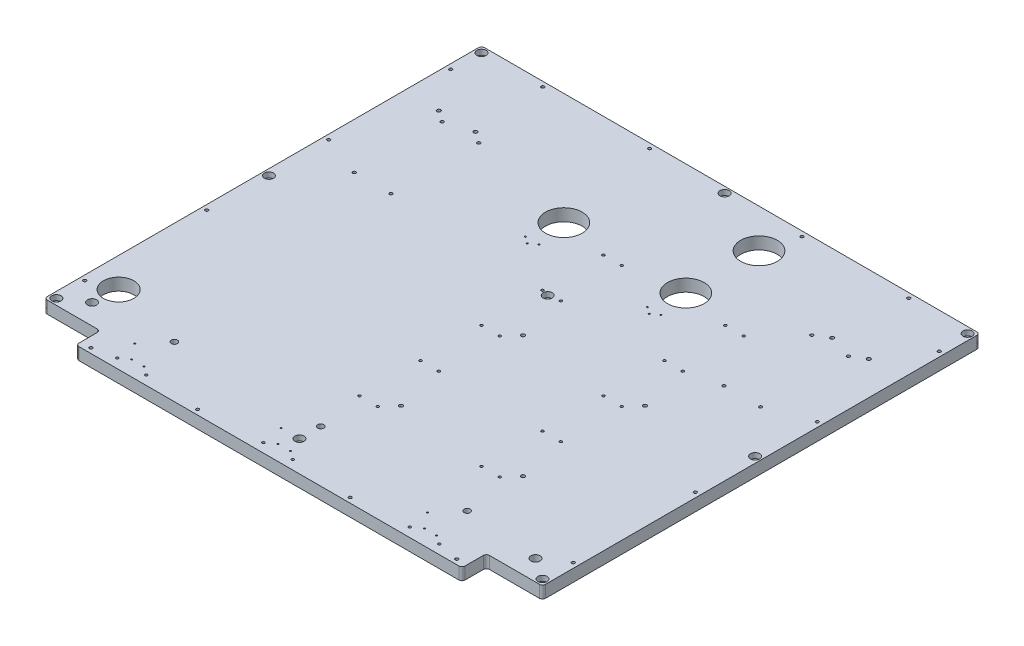
SolidWorks part; units mm, degrees
ref_plane "前视" through (0, 0, 0) normal (0, 0, 1) x (1, 0, 0)
ref_plane "上视" through (0, 0, 0) normal (0, 1, 0) x (1, 0, 0)
ref_plane "右视" through (0, 0, 0) normal (1, 0, 0) x (0, 0, -1)
sketch "草图1" plane through (0, 0, 0) normal (0, 1, 0) x (1, 0, 0)
  line L1 (-425, -375) -> (425, -375)
  line L2 (-425, -375) -> (-425, 375)
  line L3 (-425, 375) -> (425, 375)
  line L4 (425, -375) -> (425, 375)
  line L5 (-425, -375) -> (425, 375) construction
  line L6 (-425, 375) -> (425, -375) construction
  point P0 (0, 0)
  dimension "D1" = 750
  dimension "D2" = 850
extrude "凸台-拉伸1" add sketch "草图1" along normal blind 20
sketch "草图48" plane through (0, 20, 0) normal (0, 1, 0) x (1, 0, 0)
  line L0 (425, 375) -> (-425, 375) construction
  line L2 (425, -375) -> (425, 375) construction
  circle A0 centre (-90, 175) radius 30
  circle A1 centre (110, 175) radius 30
  circle A2 centre (110, 295) radius 30
  dimension "D1" = 200
  dimension "D2" = 315
  dimension "D3" = 60
  dimension "D4" = 200
  dimension "D5" = 80
extrude "切除-拉伸13" cut sketch "草图48" against normal up to next
sketch "草图47" plane through (0, 20, 0) normal (0, 1, 0) x (1, 0, 0)
  line L0 (-425, -375) -> (425, -375) construction
  line L1 (-425, 375) -> (-425, -375) construction
  circle A0 centre (-360, -285) radius 25
  dimension "D1" = 50
  dimension "D2" = 90
  dimension "D3" = 65
extrude "切除-拉伸12" cut sketch "草图47" against normal up to next
sketch "草图37" plane through (0, 20, 0) normal (0, -1, 0) x (-1, 0, 0)
  line L0 (-425, -375) -> (-425, 375) construction
  line L1 (-425, 375) -> (425, 375) construction
  line L2 (425, 375) -> (425, -375) construction
  line L3 (425, -375) -> (-425, -375) construction
  line L4 (-425, -375) -> (-425, 375)
  line L5 (-425, 375) -> (425, 375)
  line L6 (425, 375) -> (425, -375)
  line L7 (425, -375) -> (-425, -375)
  line L8 (-408.5, -358.5) -> (-408.5, 358.5)
  line L9 (-408.5, 358.5) -> (408.5, 358.5)
  line L10 (408.5, 358.5) -> (408.5, -358.5)
  line L11 (408.5, -358.5) -> (-408.5, -358.5)
  dimension "D1" = 16.5
extrude "切除-拉伸10" cut sketch "草图37" along normal through all
sketch "草图38" plane through (0, 20, 0) normal (0, 1, 0) x (1, 0, 0)
  line L1 (-316.5, -398.5) -> (316.5, -398.5)
  line L2 (-316.5, -398.5) -> (-316.5, -358.5)
  line L3 (-316.5, -358.5) -> (316.5, -358.5)
  line L4 (316.5, -398.5) -> (316.5, -358.5)
  line L5 (0, 0) -> (0, 281.3939) construction
  line L6 (408.5, -358.5) -> (-408.5, -358.5) construction
  dimension "D1" = 633
  dimension "D2" = 40
extrude "凸台-拉伸2" add sketch "草图38" against normal up to surface (20 mm away) up to face at (0, 0, 0)
sketch "草图56" plane through (0, 20, 0) normal (0, 1, 0) x (1, 0, 0)
  line L0 (0, 0) -> (0, -181.294) construction
  line L1 (-408.5, -358.5) -> (-408.5, 358.5) construction
  line L3 (-316.5, -358.5) -> (-408.5, -358.5) construction
  circle A0 centre (-363.5, -325) radius 7.5
  circle A1 centre (363.5, -325) radius 7.5
  dimension "D2" = 33.5
  dimension "D3" = 15
  dimension "D1" = 45
extrude "切除-拉伸14" cut sketch "草图56" against normal up to next
hole_wizard "M8 六角凹头螺钉的柱形沉头孔2" positions "草图46" profile "草图45" counterbore size "M8" standard "Iso" end condition through all
sketch "草图46" plane through (0, 20, 0) normal (0, 1, 0) x (1, 0, 0)
  line L0 (0, 0) -> (0, 358.5) construction
  line L4 (0, 0) -> (408.5, 0) construction
  line L6 (408.5, 358.5) -> (408.5, -358.5) construction
  line L7 (-408.5, 358.5) -> (408.5, 358.5) construction
  point P0 (-398.5, 348.5)
  point P2 (-398.5, 0)
  point P4 (-398.5, -348.5)
  point P6 (0, -348.5)
  point P8 (398.5, -348.5)
  point P10 (398.5, 0)
  point P12 (398.5, 348.5)
  point P29 (0, 348.5)
  point P32 (0, 58.5)
  dimension "D1" = 797
  dimension "D2" = 697
  dimension "D3" = 58.5
sketch "草图45" plane through (-398.5, 20, -348.5) normal (1, 0, 0) x (0, 0, 1)
  line L0 (0, 0) -> (0, 20.0001)
  line L1 (0, 20.0001) -> (4.5, 20.0001)
  line L3 (4.5, 20.0001) -> (4.5, 8.6)
  line L4 (4.5, 8.6) -> (7.5, 8.6)
  line L5 (7.5, 8.6) -> (7.5, 0)
  line L7 (7.5, 0) -> (0, 0)
  line L11 (0, -6.35) -> (0, 107.95) construction
  dimension "通孔孔直径" = 9
  dimension "通孔孔深度" = 20.0001
  dimension "柱形沉头孔直径" = 15
  dimension "柱形沉头孔深度" = 8.6
hole_wizard "M5 螺纹孔2" positions "草图40" profile "草图39" tap size "M5" standard "Iso"
sketch "草图40" plane through (0.6526, 20, 1.9724) normal (0, -1, 0) x (-1, 0, 0)
  line L0 (0.6526, 1.9724) -> (0.6526, 360.4724) construction
  line L2 (-239.3474, 360.4724) -> (-239.3474, -191.643) construction
  line L4 (240.6526, -191.643) -> (240.6526, 360.4724) construction
  line L7 (317.1526, -396.5276) -> (-315.8474, -396.5276) construction
  line L8 (409.1526, 360.4724) -> (-407.8474, 360.4724) construction
  point P0 (-215.3474, -381.5276)
  point P2 (-263.3474, -381.5276)
  point P4 (24.6526, -381.5276)
  point P6 (-23.3474, -381.5276)
  point P8 (264.6526, -381.5276)
  point P10 (216.6526, -381.5276)
  dimension "D1" = 48
  dimension "D2" = 48
  dimension "D3" = 15
  dimension "D4" = 480
sketch "草图39" plane through (216, 20, 383.5) normal (1, 0, 0) x (0, 0, 1)
  line L0 (0, 0) -> (0, 13.6618)
  line L1 (0, 13.6618) -> (2.1, 12.4)
  line L2 (2.1, 12.4) -> (2.1, 0)
  line L5 (2.1, 0) -> (0, 0)
  line L10 (0, 13.6618) -> (-2.1, 12.4) construction
  line L11 (0, -6.35) -> (0, 107.95) construction
  dimension "螺纹孔钻头直径" = 4.2
  dimension "螺纹孔钻头深度" = 12.4
  dimension "导头角度" = 118
cosmetic thread "孔螺蚊线82" parameters "D1"=10, "D2"=5
cosmetic thread "孔螺蚊线83" parameters "D1"=10, "D2"=5
cosmetic thread "孔螺蚊线84" parameters "D1"=10, "D2"=5
cosmetic thread "孔螺蚊线85" parameters "D1"=10, "D2"=5
cosmetic thread "孔螺蚊线86" parameters "D1"=10, "D2"=5
cosmetic thread "孔螺蚊线87" parameters "D1"=10, "D2"=5
hole_wizard "M3 螺纹孔3" positions "草图42" profile "草图41" tap size "M3" standard "Iso"
sketch "草图42" plane through (-240.4559, 20, 219.8338) normal (0, -1, 0) x (-1, 0, 0)
  line L0 (-456.4559, -163.6662) -> (-504.4559, -163.6662) construction
  line L2 (-480.4559, -163.6662) -> (-480.4559, 367.789) construction
  line L4 (-216.4559, -163.6662) -> (-264.4559, -163.6662) construction
  line L6 (-240.4559, -163.6662) -> (-240.4559, 379.6475) construction
  line L8 (23.5441, -163.6662) -> (-24.4559, -163.6662) construction
  line L10 (-0.4559, -163.6662) -> (-0.4559, 375.9875) construction
  line L11 (76.0441, -178.6662) -> (-556.9559, -178.6662) construction
  point P0 (9.5441, -153.6662)
  point P2 (-10.4559, -153.6662)
  point P4 (-230.4559, -153.6662)
  point P6 (-250.4559, -153.6662)
  point P8 (-470.4559, -153.6662)
  point P10 (-490.4559, -153.6662)
  point P41 (29.5441, -128.6662)
  point P43 (-210.4559, -128.6662)
  point P45 (-450.4559, -128.6662)
  dimension "D1" = 20
  dimension "D2" = 20
  dimension "D3" = 20
  dimension "D4" = 10
  dimension "D5" = 30
  dimension "D6" = 30
  dimension "D7" = 30
  dimension "D8" = 50
sketch "草图41" plane through (-250, 20, 373.5) normal (1, 0, 0) x (0, 0, 1)
  line L0 (0, 0) -> (0, 8.2511)
  line L1 (0, 8.2511) -> (1.25, 7.5)
  line L2 (1.25, 7.5) -> (1.25, 0)
  line L5 (1.25, 0) -> (0, 0)
  line L10 (0, 8.2511) -> (-1.25, 7.5) construction
  line L11 (0, -6.35) -> (0, 107.95) construction
  dimension "螺纹孔钻头直径" = 2.5
  dimension "螺纹孔钻头深度" = 7.5
  dimension "导头角度" = 118
cosmetic thread "孔螺蚊线88" parameters "D1"=6, "D2"=3
cosmetic thread "孔螺蚊线89" parameters "D1"=6, "D2"=3
cosmetic thread "孔螺蚊线90" parameters "D1"=6, "D2"=3
cosmetic thread "孔螺蚊线91" parameters "D1"=6, "D2"=3
cosmetic thread "孔螺蚊线92" parameters "D1"=6, "D2"=3
cosmetic thread "孔螺蚊线93" parameters "D1"=6, "D2"=3
cosmetic thread "孔螺蚊线123" parameters "D1"=6, "D2"=3
cosmetic thread "孔螺蚊线124" parameters "D1"=6, "D2"=3
cosmetic thread "孔螺蚊线125" parameters "D1"=6, "D2"=3
hole_wizard "Ø10.0 (10) 直径孔1" positions "草图64" profile "草图63" hole size "Ø10.0" standard "Gb" end condition up to next
sketch "草图64" plane through (0, 20, 0) normal (0, 1, 0) x (1, 0, 0)
  line L0 (216, -383.5) -> (264, -383.5) construction
  line L3 (240, -383.5) -> (240, -313.5) construction
  line L6 (-24, -383.5) -> (24, -383.5) construction
  line L9 (0, -383.5) -> (0, -313.5) construction
  line L12 (-216, -383.5) -> (-264, -383.5) construction
  line L15 (-240, -383.5) -> (-240, -313.5) construction
  point P0 (-240, -313.5)
  point P2 (0, -313.5)
  point P4 (240, -313.5)
  dimension "D1" = 70
sketch "草图63" plane through (-240, 20, 313.5) normal (1, 0, 0) x (0, 0, 1)
  line L0 (0, 0) -> (0, 20)
  line L1 (0, 20) -> (5, 20)
  line L2 (5, 20) -> (5, 0)
  line L5 (5, 0) -> (0, 0)
  line L11 (0, -6.35) -> (0, 107.95) construction
  dimension "通孔孔直径" = 10
  dimension "通孔孔深度" = 20
hole_wizard "M6 螺纹孔3" positions "草图50" profile "草图49" tap size "M6" standard "Iso" end condition up to next
sketch "草图50" plane through (0, 20, 0) normal (0, 1, 0) x (1, 0, 0)
  line L0 (0, 0) -> (408.5, 0) construction
  line L1 (408.5, 358.5) -> (408.5, -358.5) construction
  line L4 (0, 0) -> (0, 358.5) construction
  line L5 (-408.5, 358.5) -> (408.5, 358.5) construction
  line L8 (-316.5, -398.5) -> (316.5, -398.5) construction
  point P0 (-300, 350.5)
  point P2 (-125, 350.5)
  point P4 (125, 350.5)
  point P6 (300, 350.5)
  point P8 (-300, -390.5)
  point P10 (-125, -390.5)
  point P12 (125, -390.5)
  point P14 (300, -390.5)
  point P16 (-400.5, 300)
  point P18 (-400.5, 100)
  point P20 (-400.5, -100)
  point P22 (-400.5, -300)
  point P24 (400.5, 300)
  point P26 (400.5, 100)
  point P28 (400.5, -100)
  point P30 (400.5, -300)
  dimension "D1" = 250
  dimension "D2" = 600
  dimension "D3" = 8
  dimension "D4" = 200
  dimension "D5" = 600
  dimension "D6" = 8
  dimension "D7" = 250
  dimension "D8" = 600
  dimension "D9" = 8
cosmetic thread "孔螺蚊线98" parameters "D2"=6
cosmetic thread "孔螺蚊线99" parameters "D2"=6
cosmetic thread "孔螺蚊线100" parameters "D2"=6
cosmetic thread "孔螺蚊线101" parameters "D2"=6
cosmetic thread "孔螺蚊线102" parameters "D2"=6
cosmetic thread "孔螺蚊线103" parameters "D2"=6
cosmetic thread "孔螺蚊线104" parameters "D2"=6
cosmetic thread "孔螺蚊线105" parameters "D2"=6
cosmetic thread "孔螺蚊线106" parameters "D2"=6
cosmetic thread "孔螺蚊线107" parameters "D2"=6
cosmetic thread "孔螺蚊线108" parameters "D2"=6
cosmetic thread "孔螺蚊线109" parameters "D2"=6
cosmetic thread "孔螺蚊线110" parameters "D2"=6
cosmetic thread "孔螺蚊线111" parameters "D2"=6
cosmetic thread "孔螺蚊线112" parameters "D2"=6
cosmetic thread "孔螺蚊线113" parameters "D2"=6
sketch "草图49" plane through (-300, 20, -350.5) normal (1, 0, 0) x (0, 0, 1)
  line L0 (0, 0) -> (0, 20)
  line L1 (0, 20) -> (2.5, 20)
  line L2 (2.5, 20) -> (2.5, 0)
  line L5 (2.5, 0) -> (0, 0)
  line L11 (0, -6.35) -> (0, 107.95) construction
  dimension "通孔螺纹孔钻头直径" = 5
  dimension "通孔螺纹孔钻头深度" = 20
hole_wizard "M6 螺纹孔4" positions "草图58" profile "草图57" tap size "M6" standard "Iso" end condition up to next
sketch "草图58" plane through (0, 20, 0) normal (0, 1, 0) x (1, 0, 0)
  line L1 (273, 218.5) -> (333, 218.5) construction
  line L2 (273, 218.5) -> (273, 74.5) construction
  line L3 (273, 74.5) -> (333, 74.5) construction
  line L4 (333, 218.5) -> (333, 74.5) construction
  line L5 (-408.5, 358.5) -> (408.5, 358.5) construction
  line L8 (-333, 218.5) -> (-273, 218.5) construction
  line L9 (-333, 218.5) -> (-333, 74.5) construction
  line L10 (-333, 74.5) -> (-273, 74.5) construction
  line L11 (-273, 218.5) -> (-273, 74.5) construction
  line L12 (0, 358.5) -> (0, 121.2106) construction
  line L13 (-408.5, 358.5) -> (408.5, 358.5) construction
  point P0 (333, 218.5)
  point P2 (273, 218.5)
  point P4 (273, 74.5)
  point P6 (333, 74.5)
  point P130 (-333, 218.5)
  point P132 (-273, 218.5)
  point P134 (-333, 74.5)
  point P136 (-273, 74.5)
  dimension "D1" = 60
  dimension "D2" = 144
  dimension "D3" = 140
  dimension "D5" = 606
cosmetic thread "孔螺蚊线115" parameters "D2"=6
cosmetic thread "孔螺蚊线116" parameters "D2"=6
cosmetic thread "孔螺蚊线117" parameters "D2"=6
cosmetic thread "孔螺蚊线118" parameters "D2"=6
cosmetic thread "孔螺蚊线119" parameters "D2"=6
cosmetic thread "孔螺蚊线120" parameters "D2"=6
cosmetic thread "孔螺蚊线121" parameters "D2"=6
cosmetic thread "孔螺蚊线122" parameters "D2"=6
sketch "草图57" plane through (333, 20, -218.5) normal (1, 0, 0) x (0, 0, 1)
  line L0 (0, 0) -> (0, 20)
  line L1 (0, 20) -> (2.5, 20)
  line L2 (2.5, 20) -> (2.5, 0)
  line L5 (2.5, 0) -> (0, 0)
  line L11 (0, -6.35) -> (0, 107.95) construction
  dimension "通孔螺纹孔钻头直径" = 5
  dimension "通孔螺纹孔钻头深度" = 20
hole_wizard "M5 螺纹孔3" positions "草图52" profile "草图51" tap size "M5" standard "Iso" end condition up to next
sketch "草图52" plane through (0, 20, 0) normal (0, 1, 0) x (1, 0, 0)
  line L0 (-316.5, -398.5) -> (316.5, -398.5) construction
  line L1 (408.5, 358.5) -> (408.5, -358.5) construction
  point P0 (218.5, -238.5)
  dimension "D1" = 160
  dimension "D2" = 190
cosmetic thread "孔螺蚊线114" parameters "D2"=5
sketch "草图51" plane through (218.5, 20, 238.5) normal (1, 0, 0) x (0, 0, 1)
  line L0 (0, 0) -> (0, 20.001)
  line L1 (0, 20.001) -> (2.1, 20.001)
  line L2 (2.1, 20.001) -> (2.1, 0)
  line L5 (2.1, 0) -> (0, 0)
  line L11 (0, -6.35) -> (0, 107.95) construction
  dimension "通孔螺纹孔钻头直径" = 4.2
  dimension "通孔螺纹孔钻头深度" = 20.001
pattern_linear "阵列(线性)4" count 2 spacing 30 along (-1, 0, 0) count 5 spacing 100 along (0, 0, -1) of "M5 螺纹孔3"
pattern_linear "阵列(线性)5" count 2 spacing 200 along (-1, 0, 0) of "阵列(线性)4", "M5 螺纹孔3"
hole_wizard "Ø6.0 (6) 直径孔1" positions "草图54" profile "草图53" hole size "Ø6.0" standard "Gb"
sketch "草图54" plane through (0, 20, 0) normal (0, 1, 0) x (1, 0, 0)
  line L1 (-316.5, -398.5) -> (316.5, -398.5) construction
  circle A1 centre (218.5, 61.5) radius 2.1 construction
  circle A2 centre (18.5, -38.5) radius 2.1 construction
  point P0 (236.5, -18.5)
  point P2 (236.5, -218.5)
  point P4 (36.5, -18.5)
  point P6 (36.5, -218.5)
  dimension "D1" = 18
  dimension "D2" = 18
  dimension "D3" = 200
  dimension "D4" = 180
sketch "草图53" plane through (236.5, 20, 18.5) normal (1, 0, 0) x (0, 0, 1)
  line L0 (0, 0) -> (0, 16.8026)
  line L1 (0, 16.8026) -> (3, 15)
  line L2 (3, 15) -> (3, 0)
  line L5 (3, 0) -> (0, 0)
  line L10 (0, 16.8026) -> (-3, 15) construction
  line L11 (0, -6.35) -> (0, 107.95) construction
  dimension "孔直径" = 6
  dimension "孔深度" = 15
  dimension "导头角度" = 118
hole_wizard "Ø6.0 (6) 直径孔2" positions "草图60" profile "草图59" hole size "Ø6.0" standard "Gb"
sketch "草图60" plane through (0, 20, 0) normal (0, 1, 0) x (1, 0, 0)
  line L0 (408.5, 358.5) -> (408.5, -358.5) construction
  circle A1 centre (333, 218.5) radius 2.5 construction
  point P0 (-351.5, 231.5)
  point P2 (-291.5, 231.5)
  point P4 (293.5, 231.5)
  point P6 (353.5, 231.5)
sketch "草图59" plane through (-351.5, 20, -231.5) normal (1, 0, 0) x (0, 0, 1)
  line L0 (0, 0) -> (0, 11.8026)
  line L1 (0, 11.8026) -> (3, 10)
  line L2 (3, 10) -> (3, 0)
  line L5 (3, 0) -> (0, 0)
  line L10 (0, 11.8026) -> (-3, 10) construction
  line L11 (0, -6.35) -> (0, 107.95) construction
  dimension "孔直径" = 6
  dimension "孔深度" = 10
  dimension "导头角度" = 118
hole_wizard "M3 螺纹孔4" positions "草图70" profile "草图69" tap size "M3" standard "Iso"
sketch "草图70" plane through (0, 20, 0) normal (0, 1, 0) x (1, 0, 0)
  line L0 (120.5, 123.5) -> (98.5, 123.5) construction
  line L3 (109.5, 123.5) -> (109.5, 115.5) construction
  line L6 (-79.5, 123.5) -> (-101.5, 123.5) construction
  line L9 (-90.5, 123.5) -> (-90.5, 115.5) construction
  circle A0 centre (188.5, 61.5) radius 2.1 construction
  circle A1 centre (188.5, 161.5) radius 2.1 construction
  circle A2 centre (-11.5, 61.5) radius 2.1 construction
  point P0 (98.5, 123.5)
  point P2 (120.5, 123.5)
  point P4 (109.5, 115.5)
  point P6 (-101.5, 123.5)
  point P8 (-79.5, 123.5)
  point P10 (-90.5, 115.5)
  dimension "D1" = 22
  dimension "D2" = 68
  dimension "D3" = 38
  dimension "D4" = 8
  dimension "D5" = 68
sketch "草图69" plane through (98.5, 20, -123.5) normal (1, 0, 0) x (0, 0, 1)
  line L0 (0, 0) -> (0, 8.2511)
  line L1 (0, 8.2511) -> (1.25, 7.5)
  line L2 (1.25, 7.5) -> (1.25, 0)
  line L5 (1.25, 0) -> (0, 0)
  line L10 (0, 8.2511) -> (-1.25, 7.5) construction
  line L11 (0, -6.35) -> (0, 107.95) construction
  dimension "螺纹孔钻头直径" = 2.5
  dimension "螺纹孔钻头深度" = 7.5
  dimension "导头角度" = 118
cosmetic thread "孔螺蚊线128" parameters "D1"=6, "D2"=3
cosmetic thread "孔螺蚊线129" parameters "D1"=6, "D2"=3
cosmetic thread "孔螺蚊线130" parameters "D1"=6, "D2"=3
cosmetic thread "孔螺蚊线131" parameters "D1"=6, "D2"=3
cosmetic thread "孔螺蚊线132" parameters "D1"=6, "D2"=3
cosmetic thread "孔螺蚊线133" parameters "D1"=6, "D2"=3
fillet "圆角1" radius 5 8 edges at (-408.5, 10, 358.5) (408.5, 10, 358.5) (408.5, 10, -358.5) (-408.5, 10, -358.5) (-316.5, 10, 398.5) (316.5, 10, 398.5)
equation "\"D4@草图60\"=\"D1@草图60\""
